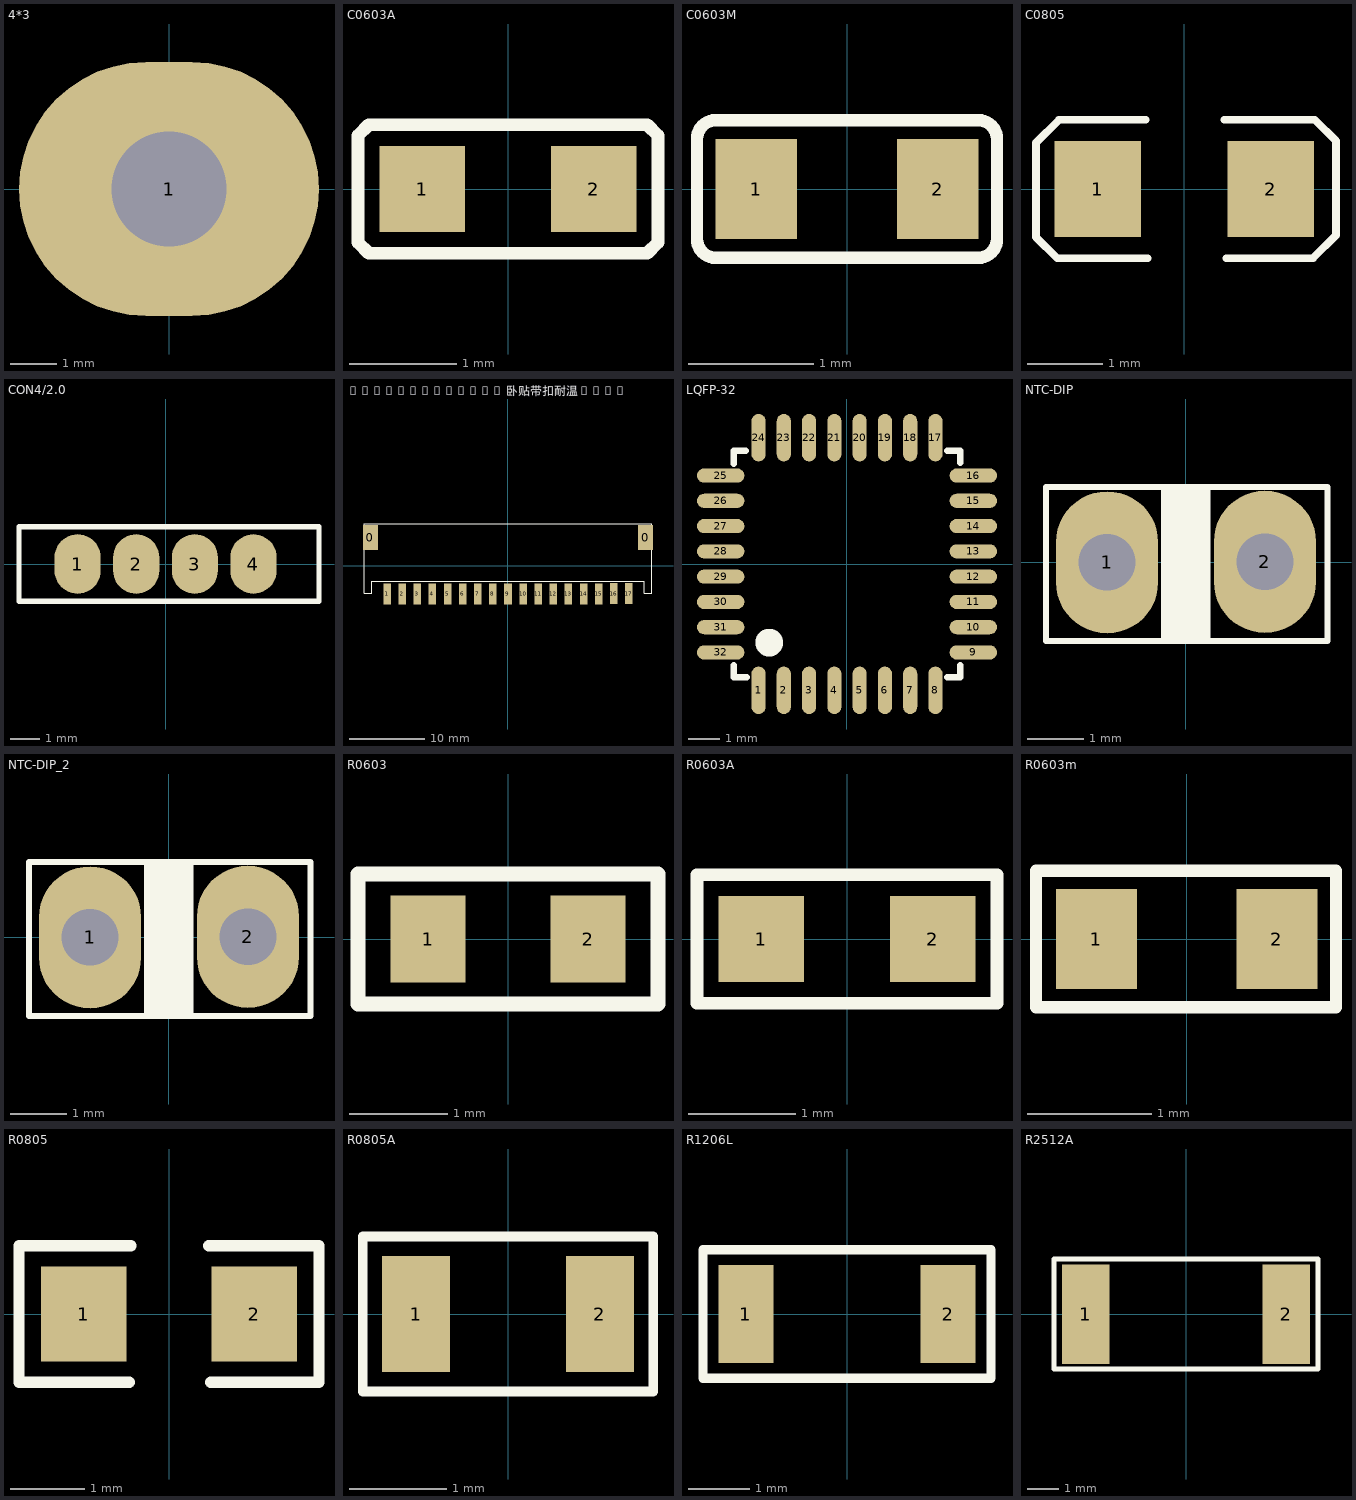
[diagram p0: the footprints below, top view; thin cyan lines are the x and y axes]
# Altium footprint library MISC86327.PcbLib: 30 footprints (part 1 of 2)
Each footprint in its own frame and in the unit in brackets; x right, y up, seen from the top. Pads: shape width x height; smd on the part's side, far side on the other; paste and mask are expansions set on the pad; w line width, h text height; cw(c..) or ccw(c..) is an arc to the next point about the centre after c.

## 4*3 [mm] "through-hole pad"
pads (1):
  oval 6.5x5.5 hole 2.5 mask+0: 1(0,0)

## C0603A [mm] "chip capacitor"
pads (2):
  rect 0.8x0.8 smd mask+0.08: 1(-0.8,0) 2(0.8,0)
Top Overlay:
  lines w0.12: 0.551,-0.6 1.2,-0.6 ; -1.4,-0.5 -1.4,0.5 -1.3,0.6 1.3,0.6 1.4,0.5 1.4,-0.5 1.3,-0.6 -1.3,-0.6 -1.4,-0.5

## C0603M [mm] "chip capacitor"
pads (2):
  rect 0.65x0.8 smd mask+0.05: 1(-0.725,0) 2(0.725,0)
Top Overlay:
  lines w0.1: -1.2,-0.4 ccw(c-1.05,-0.4) -1.05,-0.55 1.05,-0.55 ccw(c1.05,-0.4) 1.2,-0.4 1.2,0.4 ccw(c1.05,0.4) 1.05,0.55 -1.05,0.55 ccw(c-1.05,0.4) -1.2,0.4 -1.2,-0.4

## C0805 [mil]
pads (2):
  rect 45x50 smd: 1(-45,0) 2(45,0)
Top Overlay:
  lines w4: -61,36 -20,36 ; -59,36 -65,36 -77,24 -77,-25 -66,-36 -19,-36 ; 21,36 68,36 79,25 79,-24 67,-36 61,-36 ; 22,-36 63,-36
3D body "User Library-cap_0805-1.STEP": height 47.24, standoff 0, extent -39.37,-23.62 39.37,23.62

## CON4/2.0 [mil]
pads (4):
  oval 62x80 smd: 1(-118.11,0) 2(-39.37,0) 3(39.37,0) 4(118.11,0)
Top Overlay:
  lines w7: 204.37,-50 -196.85,-50 -196.85,50 204.37,50 ; 206.15,-50 206.15,50

## HY2.0WT-17A/P 卧贴带扣耐温260℃ [mm] "horizontal connector"
pads (19):
  rect 2x3.3 smd: 0(-18.2,3.725) 0(18.2,3.725)
  rect 1x2.8 smd: 1(-16,-3.725) 2(-14,-3.725) 3(-12,-3.725) 4(-10,-3.725) 5(-8,-3.725) 6(-6,-3.725) 7(-4,-3.725) 8(-2,-3.725) 9(0,-3.725) 10(2,-3.725) 11(4,-3.725) 12(6,-3.725) 13(8,-3.725) 14(10,-3.725) 15(12,-3.725) 16(14,-3.7) 17(16,-3.7)
Top Overlay:
  lines w0.15: -19,-3.625 -18,-3.625 -18,-2.025 18,-2.025 18,-3.625 19,-3.625 19,5.575 -19,5.575 -19,-3.625

## LQFP-32 [mm]
height 0.65
pads (32):
  oval 0.45x1.5 smd mask+0.152: 1(-2.8,-4) 2(-2,-4) 3(-1.2,-4) 4(-0.4,-4) 5(0.4,-4) 6(1.2,-4) 7(2,-4) 8(2.8,-4) 17(2.8,4) 18(2,4) 19(1.2,4) 20(0.4,4) 21(-0.4,4) 22(-1.2,4) 23(-2,4) 24(-2.8,4)
  oval 1.5x0.45 smd mask+0.152: 9(4,-2.8) 10(4,-2) 11(4,-1.2) 12(4,-0.4) 13(4,0.4) 14(4,1.2) 15(4,2) 16(4,2.8) 25(-4,2.8) 26(-4,2) 27(-4,1.2) 28(-4,0.4) 29(-4,-0.4) 30(-4,-1.2) 31(-4,-2) 32(-4,-2.8)
Top Overlay:
  circle w0.762: c-2.464,-2.489 r0.057
  lines w0.203: -3.58,-3.2 -3.58,-3.58 -3.175,-3.58 ; -3.58,3.175 -3.58,3.58 -3.2,3.58 ; 3.175,-3.58 3.58,-3.58 3.58,-3.2 ; 3.175,3.58 3.58,3.58 3.58,3.2

## NTC-DIP [mm]
pads (2):
  oval 1.8x2.5 hole 1: 1(-1.39,-0.005) 2(1.39,0.005)
Top Overlay:
  rectangle: -0.44,-1.389 0.43,1.27
  lines w0.1: -2.463,-1.389 2.49,-1.389 2.49,1.321 -2.463,1.321 -2.463,-1.389

## NTC-DIP_2 [mm]
pads (2):
  oval 1.8x2.5 hole 1: 1(-1.39,-0.005) 2(1.39,0.005)
Top Overlay:
  rectangle: -0.44,-1.389 0.43,1.27
  lines w0.1: -2.463,-1.389 -2.463,1.321 2.49,1.321 2.49,-1.389 -2.463,-1.389

## R0603 [mil]
pads (2):
  rect 30x35 smd: 1(-32,0) 2(32,0)
Top Overlay:
  lines w6: -60,-26 -60,26 60,26 60,-26 -60,-26
3D body "R0603.step": height 17.72, standoff 0, extent -31.49,-15.75 31.5,15.75

## R0603A [mm] "chip resistor"
height 0.5
pads (2):
  rect 0.8x0.8 smd mask+0.08: 1(-0.8,0) 2(0.8,0)
Top Overlay:
  lines w0.12: -1.4,-0.6 1.4,-0.6 1.4,0.6 -1.4,0.6 -1.4,-0.6

## R0603m [mm] "chip resistor"
pads (2):
  rect 0.65x0.8 smd mask+0.05: 1(-0.725,0) 2(0.725,0)
Top Overlay:
  lines w0.1: -1.21,-0.55 -1.21,0.55 ; -1.2,-0.55 1.2,-0.55 1.2,0.55 -1.2,0.55

## R0805 [mil]
pads (2):
  rect 45x50 smd: 1(-45,0) 2(45,0)
Top Overlay:
  lines w6: -21,-36 -79,-36 -79,36 -20,36 ; 21,36 79,36 79,-36 22,-36

## R0805A [mm] "chip resistor"
pads (2):
  rect 0.7x1.2 smd paste+0 mask+0.08: 1(-0.95,0) 2(0.95,0)
Top Overlay:
  lines w0.1: -1.5,-0.8 1.5,-0.8 1.5,0.8 -1.5,0.8 -1.5,-0.8

## R1206L [mm] "chip resistor"
pads (2):
  rect 0.9x1.6 smd: 1(-1.65,0) 2(1.65,0)
Top Overlay:
  lines w0.15: -2.35,-1.05 2.35,-1.05 2.35,1.05 -2.35,1.05 -2.35,-1.05

## R2512A [mm]
pads (2):
  rect 1.524x3.175 smd: 1(-3.2,0) 2(3.2,0)
Top Overlay:
  lines w0.152: -4.216,1.75 -4.216,-1.75 4.212,-1.75 4.212,1.75 ; -4.216,1.758 4.214,1.758
3D body "2512_R.step": height 0.64, standoff 0.02, extent -3.059,-1.594 3.241,1.606